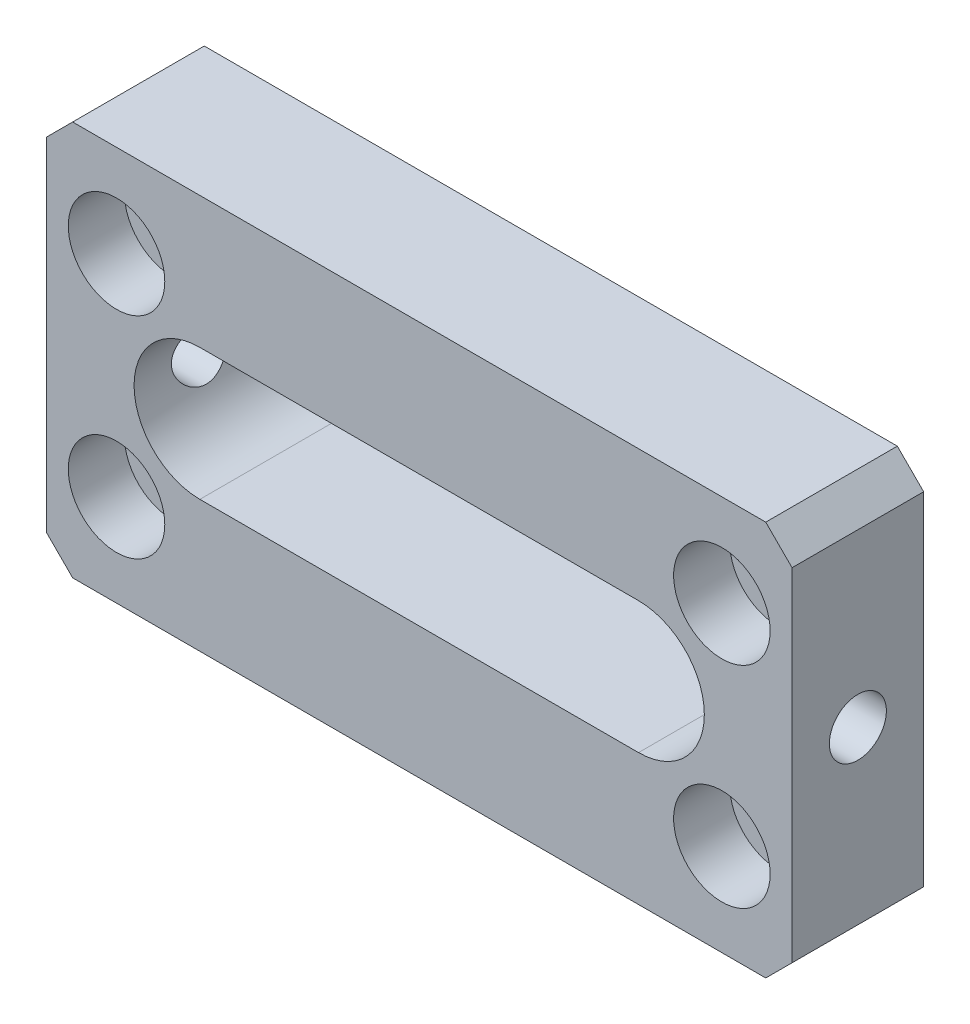
SolidWorks part; units mm, degrees
material "普通碳钢"
ref_plane "前视基准面" through (0, 0, 0) normal (0, 0, 1) x (1, 0, 0)
ref_plane "上视基准面" through (0, 0, 0) normal (0, 1, 0) x (1, 0, 0)
ref_plane "右视基准面" through (0, 0, 0) normal (1, 0, 0) x (0, 0, -1)
sketch "草图1" plane through (0, 0, 0) normal (0, 0, 1) x (1, 0, 0)
  line L0 (-25, 0) -> (25, 0) construction
  line L1 (-42.5, -22.5) -> (42.5, -22.5)
  line L2 (-42.5, -22.5) -> (-42.5, 22.5)
  line L3 (-42.5, 22.5) -> (42.5, 22.5)
  line L4 (42.5, -22.5) -> (42.5, 22.5)
  line L5 (-42.5, -22.5) -> (42.5, 22.5) construction
  line L6 (-42.5, 22.5) -> (42.5, -22.5) construction
  line L7 (-25, 7.5) -> (25, 7.5)
  line L8 (-25, -7.5) -> (25, -7.5)
  arc A0 (-25, 7.5) -> (-25, -7.5) centre (-25, 0) ccw
  arc A1 (25, -7.5) -> (25, 7.5) centre (25, 0) ccw
  point P0 (0, 0)
  point P8 (0, 0)
  dimension "D4" = 7.5
  dimension "D1" = 85
  dimension "D2" = 45
  dimension "D3" = 50
extrude "凸台-拉伸1" add sketch "草图1" along normal blind 15
hole_wizard "M6 六角凹头螺钉的柱形沉头孔1" positions "草图3" profile "草图2" counterbore size "M6" standard "Iso" end condition through all
sketch "草图3" plane through (0, 0, 15) normal (0, 0, 1) x (1, 0, 0)
  line L1 (0, 0) -> (52.1701, 0) construction
  line L3 (-47.0657, 12) -> (54.5818, 12) construction
  line L5 (0, 0) -> (0, 28.4972) construction
  line L7 (-34.5, 26.4777) -> (-34.5, -30.0679) construction
  line L9 (-51.5535, -12) -> (58.733, -12) construction
  line L11 (34.5, 29.8435) -> (34.5, -33.4337) construction
  point P77 (-34.5, 12)
  point P79 (-34.5, -12)
  point P81 (34.5, -12)
  point P83 (34.5, 12)
  dimension "D1" = 34.5
  dimension "D2" = 34.5
  dimension "D3" = 12
  dimension "D4" = 12
sketch "草图2" plane through (-34.5, 12, 15) normal (1, 0, 0) x (0, -1, 0)
  line L0 (0, 0) -> (0, 15)
  line L1 (0, 15) -> (3.3, 15)
  line L3 (3.3, 15) -> (3.3, 6.4)
  line L4 (3.3, 6.4) -> (5.5, 6.4)
  line L5 (5.5, 6.4) -> (5.5, 0)
  line L7 (5.5, 0) -> (0, 0)
  line L11 (0, -6.35) -> (0, 107.95) construction
  dimension "通孔孔直径" = 6.6
  dimension "通孔孔深度" = 15
  dimension "柱形沉头孔直径" = 11
  dimension "柱形沉头孔深度" = 6.4
sketch "草图4" plane through (-42.5, 0, 0) normal (-1, 0, 0) x (0, 0, 1)
  line L0 (0, 0) -> (15, 0) construction
  line L1 (15, 22.5) -> (15, -22.5) construction
  circle A0 centre (7.5, 0) radius 3.25
  dimension "D1" = 6.5
extrude "切除-拉伸1" cut sketch "草图4" against normal blind 162
chamfer "倒角1" distance 3 angle 45 4 edges at (42.5, -22.5, 7.5) (-42.5, -22.5, 7.5) (42.5, 22.5, 7.5) (-42.5, 22.5, 7.5)
sketch "草图5" plane through (0, 0, 15) normal (0, 0, 1) x (1, 0, 0)
  circle A0 centre (0, 0) radius 7.5
